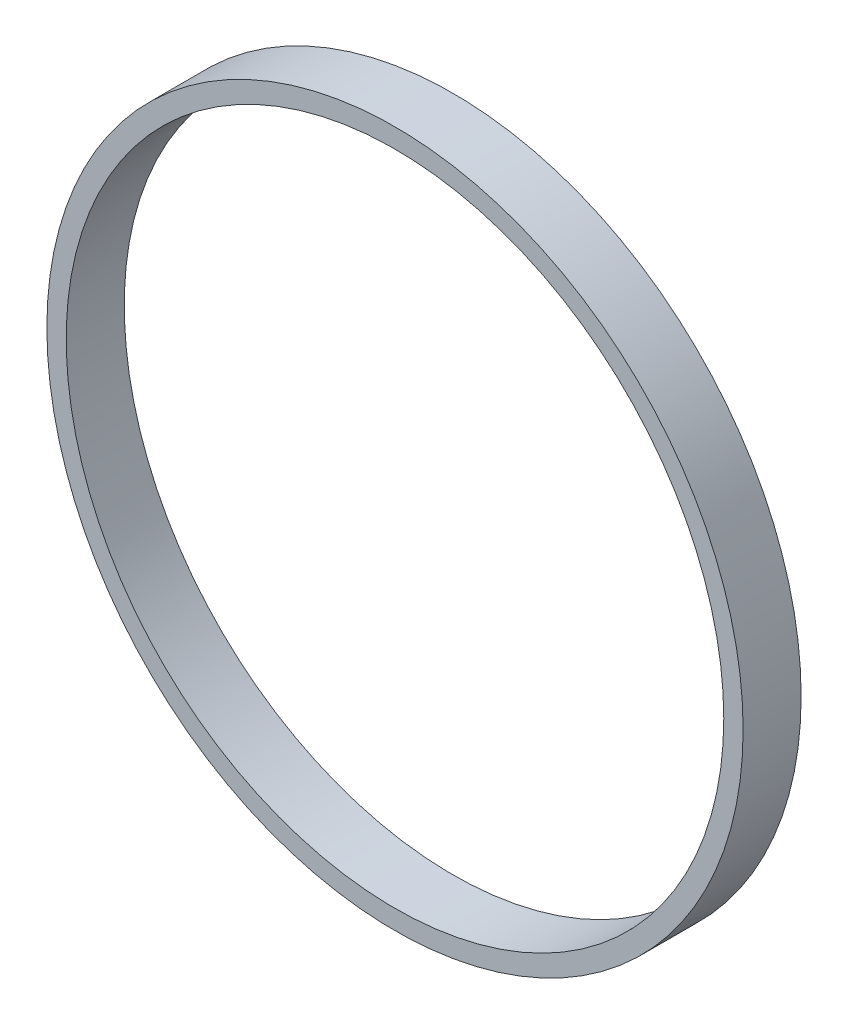
from build123d import *

# Parameters (mm, degrees)
SKETCH2_R           = 90
SKETCH2_R_2         = 85
BOSS_EXTRUDE1_DEPTH = 15


with BuildPart() as part:
    # Sketch2 → Boss-Extrude1 (new body)
    with BuildSketch(Plane.XY):
        Circle(SKETCH2_R)
        Circle(SKETCH2_R_2, mode=Mode.SUBTRACT)
    extrude(amount=BOSS_EXTRUDE1_DEPTH)


solid = part.part
